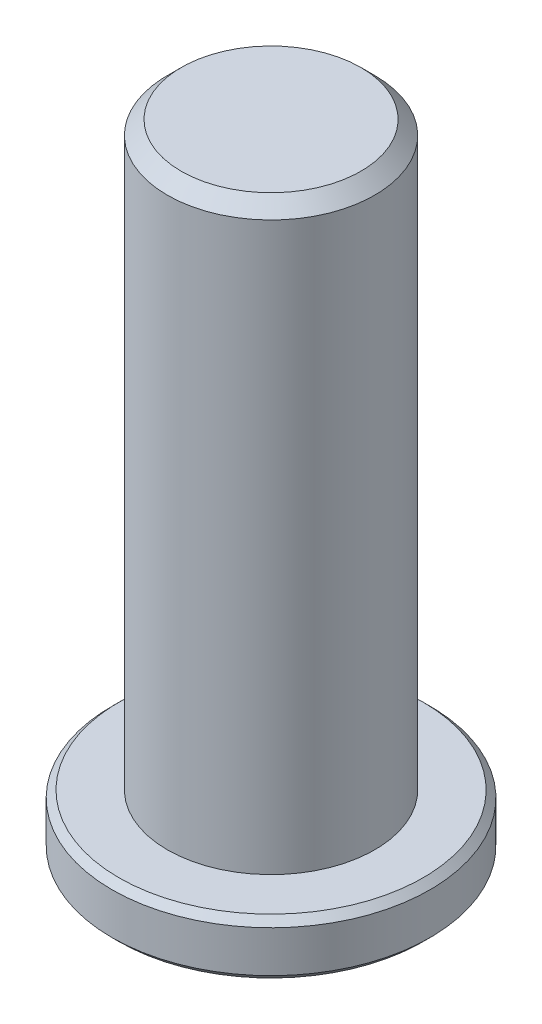
SolidWorks part; units mm, degrees
material "普通碳钢"
ref_plane "Front Plane" through (0, 0, 0) normal (0, 0, 1) x (1, 0, 0)
ref_plane "Top Plane" through (0, 0, 0) normal (0, 1, 0) x (1, 0, 0)
ref_plane "Right Plane" through (0, 0, 0) normal (1, 0, 0) x (0, 0, -1)
sketch "Sketch1" plane through (0, 0, 0) normal (0, 1, 0) x (1, 0, 0)
  circle A0 centre (0, 0) radius 11.5
  dimension "D1" = 23
extrude "Boss-Extrude1" add sketch "Sketch1" along normal blind 4
sketch "Sketch2" plane through (0, 4, 0) normal (0, 1, 0) x (1, 0, 0)
  circle A0 centre (0, 0) radius 7.5
  dimension "D1" = 15
extrude "Boss-Extrude2" add sketch "Sketch2" along normal blind 42
chamfer "Chamfer1" distance 1 angle 45 1 edges at (0, 46, 7.5)
chamfer "Chamfer2" distance 0.5 angle 45 2 edges at (0, 0, 11.5) (0, 4, 11.5)
